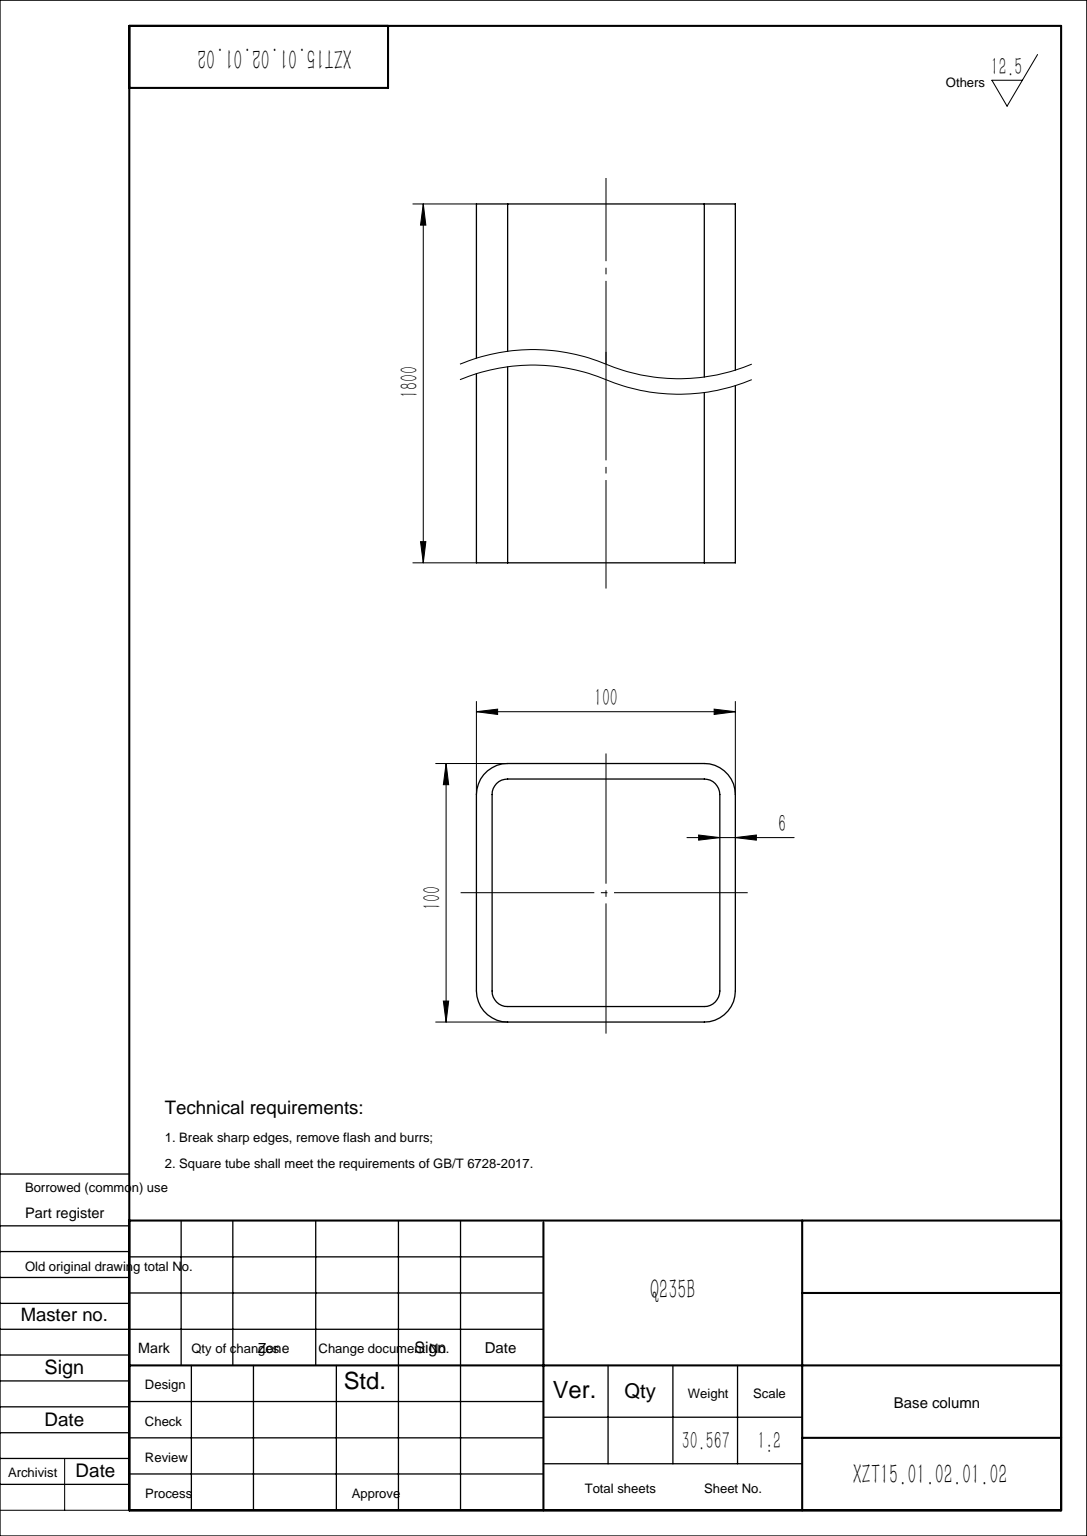
from build123d import *

# Parameters (mm, degrees)
GB_T_6728_2002_SQUARE_HOLLOW_SECTION_100_DEPTH = 1800


with BuildPart() as part:
    # Sketch11 → GB/T 6728-2002 square hollow section 100×100×6(1) (new body)
    with BuildSketch(Plane(origin=(0, 0, 0), x_dir=(-1, 0, 0), z_dir=(0, 1, 0))):
        with BuildLine():
            Line((-38, -50), (38, -50))
            ThreePointArc((38, -50), (46.485281374, -46.485281374), (50, -38))
            Line((50, -38), (50, 38))
            ThreePointArc((50, 38), (46.485281374, 46.485281374), (38, 50))
            Line((38, 50), (-38, 50))
            ThreePointArc((-38, 50), (-46.485281374, 46.485281374), (-50, 38))
            Line((-50, 38), (-50, -38))
            ThreePointArc((-50, -38), (-46.485281374, -46.485281374), (-38, -50))
        make_face()
        with BuildLine():
            Line((-38, -44), (38, -44))
            ThreePointArc((38, -44), (42.242640687, -42.242640687), (44, -38))
            Line((44, -38), (44, 38))
            ThreePointArc((44, 38), (42.242640687, 42.242640687), (38, 44))
            Line((38, 44), (-38, 44))
            ThreePointArc((-38, 44), (-42.242640687, 42.242640687), (-44, 38))
            Line((-44, 38), (-44, -38))
            ThreePointArc((-44, -38), (-42.242640687, -42.242640687), (-38, -44))
        make_face(mode=Mode.SUBTRACT)
    extrude(amount=GB_T_6728_2002_SQUARE_HOLLOW_SECTION_100_DEPTH)


solid = part.part
